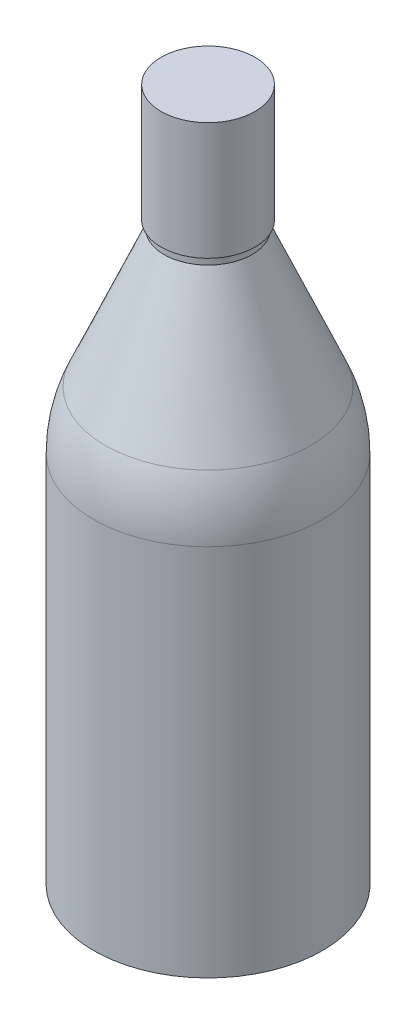
from build123d import *

# Parameters (mm, degrees)
BOSS_EXTRUDE1_START = -5
SKETCH2_R           = 7
BOSS_EXTRUDE1_DEPTH = 5
BOSS_EXTRUDE2_START = 40
SKETCH3_R           = 16
SKETCH3_R_2         = 15
BOSS_EXTRUDE2_DEPTH = 40


with BuildPart() as part:
    # Sketch1 → Revolve1 (revolve)
    with BuildSketch(Plane.XY, mode=Mode.PRIVATE) as revolve1_sk:
        with BuildLine():
            Line((0, 0), (39, 0))
            Line((39, 0), (39, 127.168593742))
            ThreePointArc((39, 127.168593742), (37.973366174, 137.248742828), (34.935623776, 146.914947034))
            Line((34.935623776, 146.914947034), (15, 193.29086769))
            Line((15, 193.29086769), (15, 236))
            Line((15, 236), (7, 236))
            Line((7, 236), (7, 191.64423404))
            Line((7, 191.64423404), (31, 135.813420404))
            Line((31, 135.813420404), (31, 8))
            Line((31, 8), (0, 8))
            Line((0, 8), (0, 0))
        make_face()
    revolve(revolve1_sk.sketch.rotate(Axis((0, 0, 0), (0, 1, 0)), 90), axis=Axis((0, 0, 0), (0, 1, 0)))

    # Sketch2 → Boss-Extrude1 (add)
    with BuildSketch(Plane(origin=(0, 236, 0), x_dir=(1, 0, 0), z_dir=(0, 1, 0)).offset(BOSS_EXTRUDE1_START)):
        with Locations(Location((0, 0, 0), (0, 0, 90))):
            Circle(SKETCH2_R)
    extrude(amount=BOSS_EXTRUDE1_DEPTH)

    # Sketch3 → Boss-Extrude2 (add)
    with BuildSketch(Plane(origin=(0, 196, 0), x_dir=(1, 0, 0), z_dir=(0, 1, 0)).offset(BOSS_EXTRUDE2_START)):
        with Locations(Location((0, 0, 0), (0, 0, 270))):
            Circle(SKETCH3_R)
        with Locations(Location((0, 0, 0), (0, 0, 90))):
            Circle(SKETCH3_R_2, mode=Mode.SUBTRACT)
    extrude(amount=-BOSS_EXTRUDE2_DEPTH)


solid = part.part
